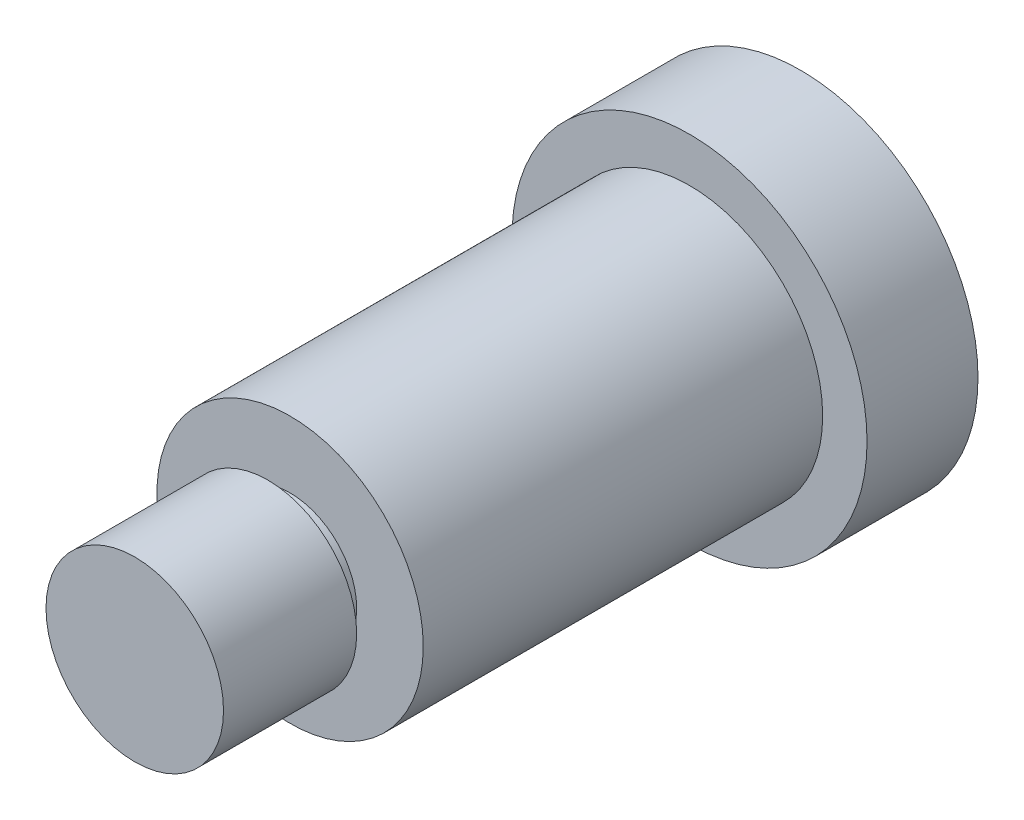
SolidWorks part; units mm, degrees
material "20#"
ref_plane "Front Plane" through (0, 0, 0) normal (0, 0, 1) x (1, 0, 0)
ref_plane "Top Plane" through (0, 0, 0) normal (0, 1, 0) x (1, 0, 0)
ref_plane "Right Plane" through (0, 0, 0) normal (1, 0, 0) x (0, 0, -1)
sketch "Sketch1" plane through (0, 0, 0) normal (1, 0, 0) x (0, 0, -1)
  line L0 (0, 0) -> (30, 0) construction
  line L1 (30, 0) -> (30, 8)
  line L2 (30, 8) -> (25, 8)
  line L3 (25, 8) -> (25, 6)
  line L4 (25, 6) -> (7, 6)
  line L5 (7, 6) -> (7, 3)
  line L6 (6, 4) -> (0, 4)
  line L7 (0, 4) -> (0, 0)
  line L8 (0, 0) -> (30, 0)
  line L9 (7, 3) -> (6, 3)
  line L10 (6, 3) -> (6, 4)
  dimension "D1" = 30
  dimension "D2" = 5
  dimension "D3" = 18
  dimension "D4" = 7
  dimension "D5" = 8
  dimension "D6" = 12
  dimension "D7" = 16
  dimension "D8" = 1
  dimension "D9" = 1
revolve "Revolve1" add sketch "Sketch1" angle 360 about L0
cosmetic thread "Cosmetic Thread1" parameters "D2"=6.647
